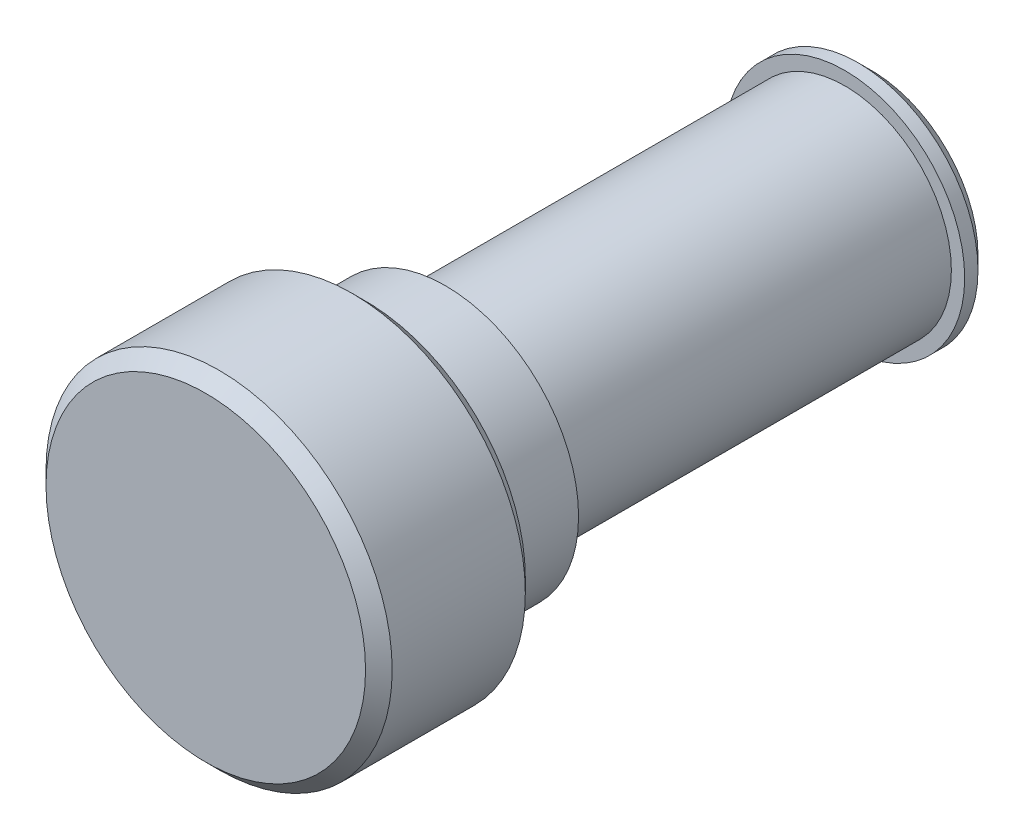
SolidWorks part; units mm, degrees
ref_plane "Front Plane" through (0, 0, 0) normal (0, 0, 1) x (1, 0, 0)
ref_plane "Top Plane" through (0, 0, 0) normal (0, 1, 0) x (1, 0, 0)
ref_plane "Right Plane" through (0, 0, 0) normal (1, 0, 0) x (0, 0, -1)
other "Configuration Table"
sketch "Sketch1" plane through (0, 0, 0) normal (0, 0, 1) x (1, 0, 0)
  circle A0 centre (0, 0) radius 4.5
  dimension "D1" = 9
extrude "Boss-Extrude1" add sketch "Sketch1" along normal blind 1
sketch "Sketch2" plane through (0, 0, 1) normal (0, 0, 1) x (1, 0, 0)
  circle A0 centre (0, 0) radius 4
  dimension "D1" = 8
extrude "Boss-Extrude2" add sketch "Sketch2" along normal blind 1
sketch "Sketch3" plane through (0, 0, 2) normal (0, 0, 1) x (1, 0, 0)
  circle A0 centre (0, 0) radius 4
  dimension "D1" = 8
extrude "Boss-Extrude3" add sketch "Sketch3" along normal blind 14
sketch "Sketch4" plane through (0, 0, 16) normal (0, 0, 1) x (1, 0, 0)
  circle A0 centre (0, 0) radius 5
  dimension "D1" = 10
extrude "Boss-Extrude4" add sketch "Sketch4" along normal blind 3
sketch "Sketch5" plane through (0, 0, 19) normal (0, 0, 1) x (1, 0, 0)
  circle A0 centre (0, 0) radius 6.5
  dimension "D1" = 13
extrude "Boss-Extrude5" add sketch "Sketch5" along normal blind 6
chamfer "Chamfer1" distance 0.5 angle 45 3 edges at (6.5, 0, 25) (4.5, 0, 0) (6.5, 0, 19)
